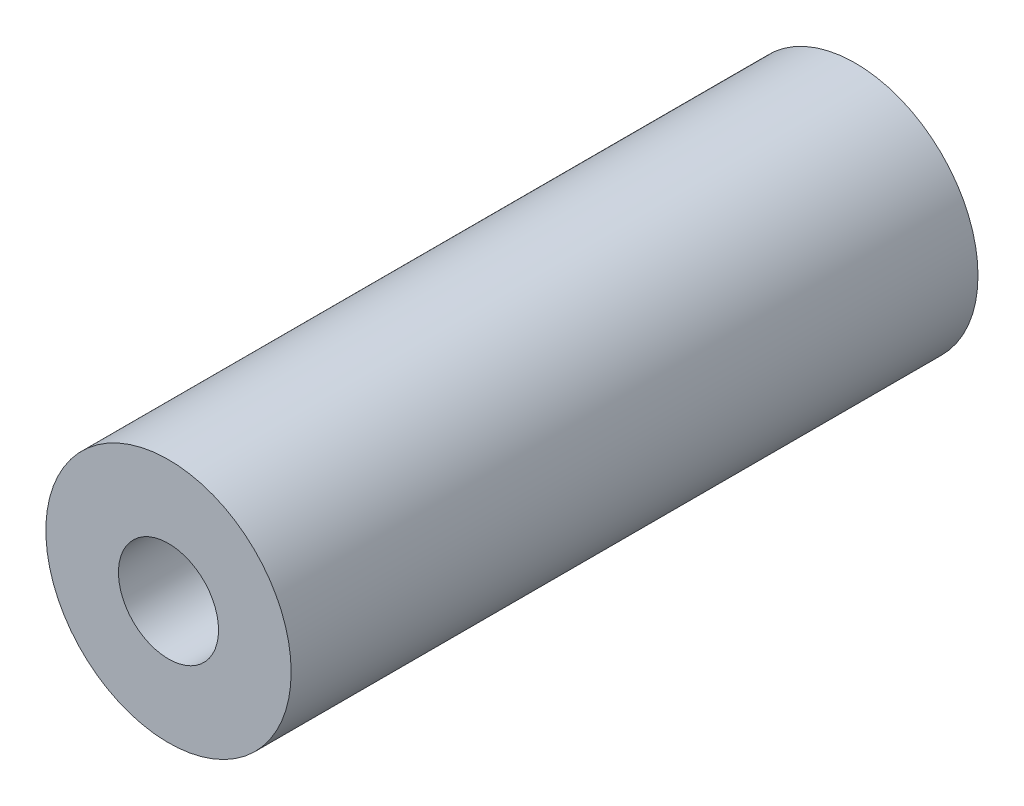
from build123d import *

# Parameters (mm, degrees)
SKETCH1_R              = 12.5
BOSS_EXTRUDE1_DEPTH    = 70
M12_TAPPED_HOLE1_D     = 10.2
M12_TAPPED_HOLE1_DEPTH = 30
M12_TAPPED_HOLE1_TIP   = 3.064389157
M12_TAPPED_HOLE2_D     = 10.2
M12_TAPPED_HOLE2_DEPTH = 30
M12_TAPPED_HOLE2_TIP   = 3.064389157


with BuildPart() as part:
    # Sketch1 → Boss-Extrude1 (new body)
    with BuildSketch(Plane.XY):
        Circle(SKETCH1_R)
    extrude(amount=BOSS_EXTRUDE1_DEPTH)

    # M12 Tapped Hole1
    with Locations(Plane.XY.offset(70)):
        with Locations((0, 0)):
            Hole(M12_TAPPED_HOLE1_D / 2, depth=M12_TAPPED_HOLE1_DEPTH)
            with Locations((0, 0, -(M12_TAPPED_HOLE1_DEPTH + M12_TAPPED_HOLE1_TIP / 2))):  # 118° drill point
                Cone(0, M12_TAPPED_HOLE1_D / 2, M12_TAPPED_HOLE1_TIP, mode=Mode.SUBTRACT)

    # M12 Tapped Hole2
    with Locations(Plane(origin=(0, 0, 0), x_dir=(-1, 0, 0), z_dir=(0, 0, -1))):
        with Locations((0, 0)):
            Hole(M12_TAPPED_HOLE2_D / 2, depth=M12_TAPPED_HOLE2_DEPTH)
            with Locations((0, 0, -(M12_TAPPED_HOLE2_DEPTH + M12_TAPPED_HOLE2_TIP / 2))):  # 118° drill point
                Cone(0, M12_TAPPED_HOLE2_D / 2, M12_TAPPED_HOLE2_TIP, mode=Mode.SUBTRACT)


solid = part.part
